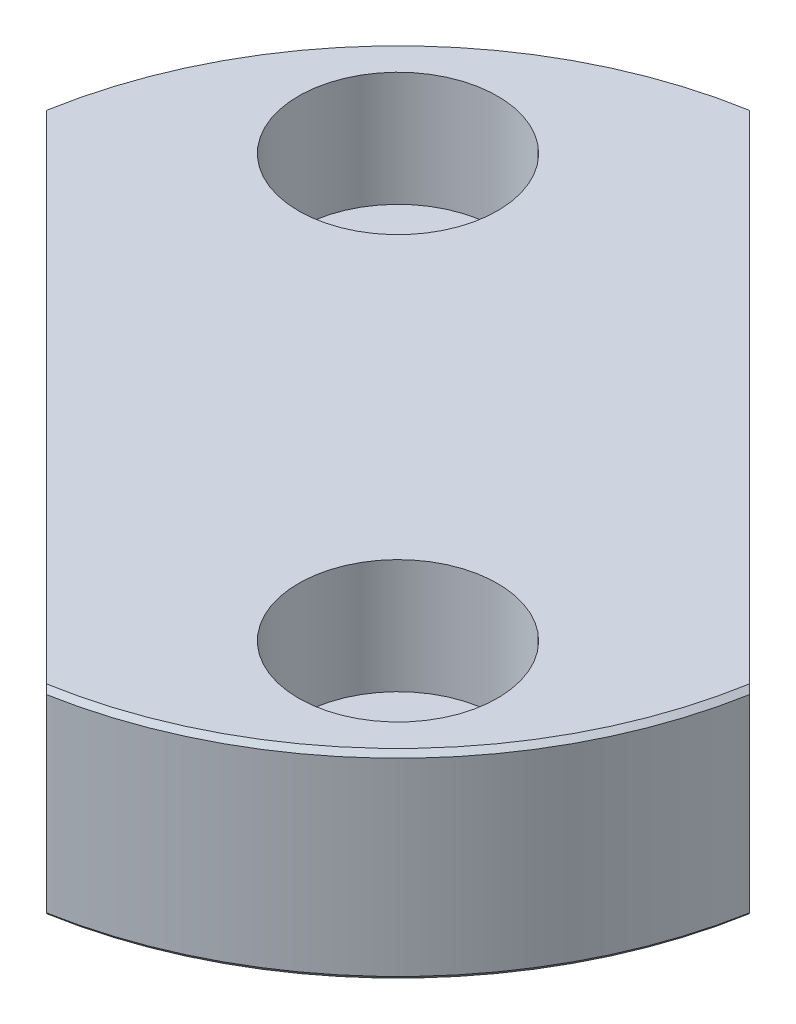
SolidWorks part; units mm, degrees
material "AISI 类型 316L 不锈钢"
ref_plane "Front Plane" through (0, 0, 0) normal (0, 0, 1) x (1, 0, 0)
ref_plane "Top Plane" through (0, 0, 0) normal (0, 1, 0) x (1, 0, 0)
ref_plane "Right Plane" through (0, 0, 0) normal (1, 0, 0) x (0, 0, -1)
sketch "Sketch2" plane through (0, 0, 0) normal (0, 0, 1) x (1, 0, 0)
  line L0 (0, 0) -> (0, 24) construction
  line L1 (0, 24) -> (-17.5, 24)
  line L2 (-17.5, 24) -> (-17.5, 16)
  line L3 (-17.5, 16) -> (-6.75, 16)
  line L4 (-6.75, 16) -> (-6.75, 0)
  line L5 (-6.75, 0) -> (0, 0)
  line L6 (0, 0) -> (0, 24)
  dimension "D1" = 35
  dimension "D2" = 13.5
  dimension "D3" = 16
  dimension "D4" = 8
revolve "Revolve1" add sketch "Sketch2" angle 360 about L0
hole_wizard "G1/8 Tapped Hole1" positions "3DSketch1" profile "Sketch4" tap size "G1/8" standard "GB" end condition up to next
sketch3d "3DSketch1"
  line L0 (0, 24, 0) -> (0, 16, 0) construction
  point P0 (0, 24, 0)
sketch "Sketch4" plane through (0, 24, 0) normal (1, 0, 0) x (0, 0, 1)
  line L0 (0, 0) -> (0, 24)
  line L1 (0, 24) -> (4.4, 24)
  line L2 (4.4, 24) -> (4.4, 0)
  line L5 (4.4, 0) -> (0, 0)
  line L11 (0, -6.35) -> (0, 107.95) construction
  dimension "通孔螺纹孔钻头直径" = 8.8
  dimension "通孔螺纹孔钻头深度" = 24
cosmetic thread "Cosmetic Thread 1" parameters "D2"=9.728
sketch "Sketch5" plane through (0, 24, 0) normal (0, 1, 0) x (1, 0, 0)
  line L0 (0, 12) -> (0, -12) construction
  line L1 (12, 0) -> (-12, 0) construction
  line L2 (0, 0) -> (-8.4853, 8.4853) construction
  line L3 (0, 0) -> (8.4853, -8.4853) construction
  circle A0 centre (0, 0) radius 12 construction
  dimension "D1" = 24
  dimension "D2" = 45
hole_wizard "Hole Size (% based on) Socket Head Cap Screw Type 1" positions "3DSketch2" profile "Sketch6" counterbore size "M4" standard "GB" end condition up to next
sketch3d "3DSketch2"
  point P13 (-8.4853, 24, -8.4853)
  point P16 (8.4853, 24, 8.4853)
sketch "Sketch6" plane through (-8.4853, 24, -8.4853) normal (1, 0, 0) x (0, 0, 1)
  line L0 (0, 0) -> (0, 8)
  line L1 (0, 8) -> (2.4, 8)
  line L3 (2.4, 8) -> (2.4, 4.6)
  line L4 (2.4, 4.6) -> (4, 4.6)
  line L5 (4, 4.6) -> (4, 0)
  line L7 (4, 0) -> (0, 0)
  line L11 (0, -6.35) -> (0, 107.95) construction
  dimension "通孔孔直径" = 4.8
  dimension "通孔孔深度" = 8
  dimension "柱形沉头孔直径" = 8
  dimension "柱形沉头孔深度" = 4.6
fillet "Fillet1" radius 0.2 1 edges at (0, 16, -6.75)
chamfer "Chamfer1" distance 0.2 angle 45 3 edges at (0, 0, -6.75) (0, 24, -17.5) (0, 16, -17.5)
chamfer "Chamfer2" distance 0.5 angle 45 2 edges at (0, 0, 4.4) (0, 24, 4.4)
sketch "Sketch7" plane through (0, 24, 0) normal (0, 1, 0) x (1, 0, 0)
  line L0 (0, 0) -> (12.2329, 12.2329) construction
  line L1 (0, 0) -> (17.3, 0) construction
  line L2 (-3.084, 17.2261) -> (17.2261, -3.084)
  line L3 (0, 0) -> (12.2329, -12.2329) construction
  line L4 (0, 12) -> (0, -12) construction
  line L5 (-17.2261, 3.084) -> (3.084, -17.2261)
  circle A0 centre (0, 0) radius 17.3 construction
  circle A1 centre (0, 0) radius 17.5 construction
  circle A2 centre (0, 0) radius 17.5
  point P9 (7.0711, 7.0711)
  circle M7 centre (0, 0) radius 17.3
  dimension "D1" = 45
  dimension "D2" = 45
  dimension "D3" = 10
extrude "Cut-Extrude1" cut sketch "Sketch7" against normal through all contours L5 M7 | L2 M7 | L5 A2 M7 | L2 A2 M7
sketch "Sketch8" plane through (0, 16, 0) normal (0, -1, 0) x (1, 0, 0)
  circle A0 centre (0, 0) radius 15
  dimension "D1" = 30
extrude "Cut-Extrude2" cut sketch "Sketch8" along normal through all
sketch "Sketch9" plane through (0, 16, 0) normal (0, -1, 0) x (1, 0, 0)
  circle A0 centre (0, 0) radius 7
  dimension "D1" = 14
extrude "Boss-Extrude1" add sketch "Sketch9" against normal up to surface (8 mm away) up to face at (-8.4853, 24, -4.4853)
